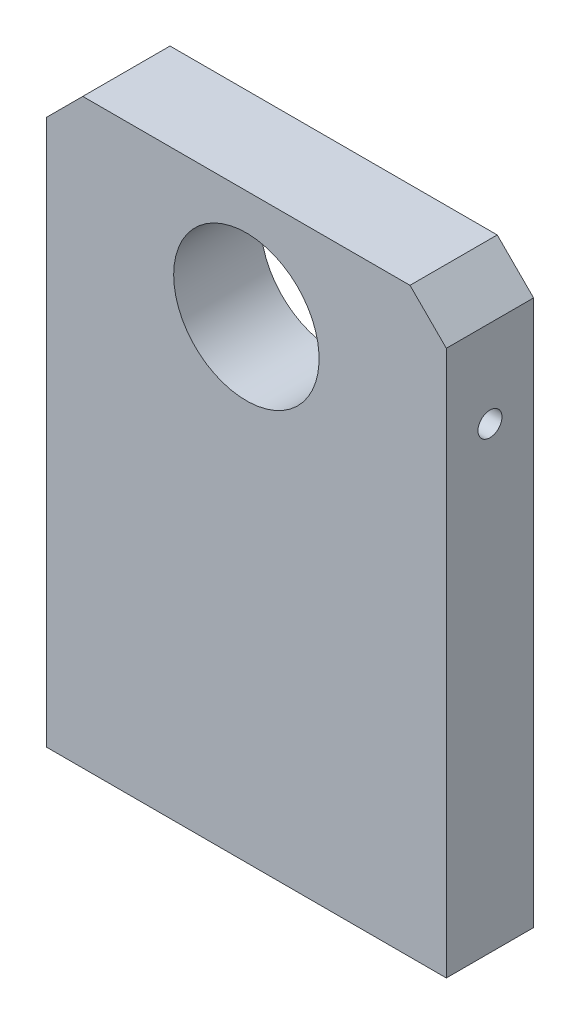
SolidWorks part; units mm, degrees
ref_plane "前视基准面" through (0, 0, 0) normal (0, 0, 1) x (1, 0, 0)
ref_plane "上视基准面" through (0, 0, 0) normal (0, 1, 0) x (1, 0, 0)
ref_plane "右视基准面" through (0, 0, 0) normal (1, 0, 0) x (0, 0, -1)
sketch "草图1" plane through (0, 0, 0) normal (0, 0, 1) x (1, 0, 0)
  line L1 (-27.5, -40) -> (27.5, -40)
  line L2 (-27.5, -40) -> (-27.5, 40)
  line L3 (-27.5, 40) -> (27.5, 40)
  line L4 (27.5, -40) -> (27.5, 40)
  line L5 (-27.5, -40) -> (27.5, 40) construction
  line L6 (-27.5, 40) -> (27.5, -40) construction
  point P0 (0, 0)
  dimension "D1" = 80
  dimension "D2" = 55
extrude "凸台-拉伸1" add sketch "草图1" along normal blind 12
sketch "草图2" plane through (0, 0, 12) normal (0, 0, 1) x (1, 0, 0)
  circle A0 centre (0, 0) radius 10.5 construction
  circle A1 centre (85, 0) radius 10
  circle A2 centre (-85, 0) radius 10
sketch "草图3" plane through (0, 0, 0) normal (0, 0, -1) x (-1, 0, 0)
  line L0 (-27.5, 40) -> (27.5, 40) construction
  line L1 (27.5, -40) -> (17.5, -40)
  line L2 (27.5, -40) -> (27.5, 40)
  line L3 (27.5, 40) -> (17.5, 40)
  line L4 (17.5, -40) -> (17.5, 40)
  line L6 (-27.5, -40) -> (-17.5, -40)
  line L7 (-27.5, -40) -> (-27.5, 40)
  line L8 (-27.5, 40) -> (-17.5, 40)
  line L9 (-17.5, -40) -> (-17.5, 40)
  dimension "D1" = 10
extrude "切除-拉伸2" [suppressed] cut sketch "草图3" against normal blind 1.5
sketch "草图4" plane through (0, 40, 0) normal (0, 1, 0) x (1, 0, 0)
  line L0 (27.5, -12) -> (-27.5, -12) construction
  line L1 (-15, 0) -> (15, 0)
  line L2 (-15, 0) -> (-15, -12)
  line L3 (-15, -12) -> (15, -12)
  line L4 (15, 0) -> (15, -12)
  line L5 (-15, 0) -> (15, -12) construction
  line L6 (-15, -12) -> (15, 0) construction
  line L7 (27.5, 0) -> (-27.5, 0) construction
  point P0 (0, -6)
  dimension "D1" = 30
extrude "切除-拉伸3" [suppressed] cut sketch "草图4" against normal blind 8
sketch "草图5" plane through (0, 0, 0) normal (0, 0, -1) x (-1, 0, 0)
  circle A0 centre (0, 25) radius 10
  dimension "D1" = 20
  dimension "D2" = 25
extrude "切除-拉伸4" cut sketch "草图5" against normal up to next
chamfer "倒角1" distance 5 angle 45 2 edges at (-27.5, 40, 6) (27.5, 40, 6)
hole_wizard "M4 螺纹孔1" positions "3D草图1" profile "草图6" tap size "M4" standard "GB"
sketch3d "3D草图1"
  line L4 (27.5, 23, 12) -> (27.5, 23, 0)
  line L5 (27.5, -40, 12) -> (27.5, 35, 12) construction
  line L6 (27.5, -40, 0) -> (27.5, 35, 0) construction
  line L8 (27.5, 35, 0) -> (27.5, 35, 12) construction
  point P0 (27.5, 23, 6)
  dimension "D1" = 12
sketch "草图6" plane through (27.5, 23, 6) normal (0, 1, 0) x (0, 0, -1)
  line L0 (0, 0) -> (0, 17.702)
  line L1 (0, 17.702) -> (1.65, 17.702)
  line L2 (1.65, 17.702) -> (1.65, 0)
  line L5 (1.65, 0) -> (0, 0)
  line L11 (0, -6.35) -> (0, 107.95) construction
  dimension "通孔螺纹孔钻头直径" = 3.3
  dimension "通孔螺纹孔钻头深度" = 17.702
cosmetic thread "孔螺蚊线1" parameters "D2"=4
equation "\"D5@草图2\"=\"D4@草图2\""
